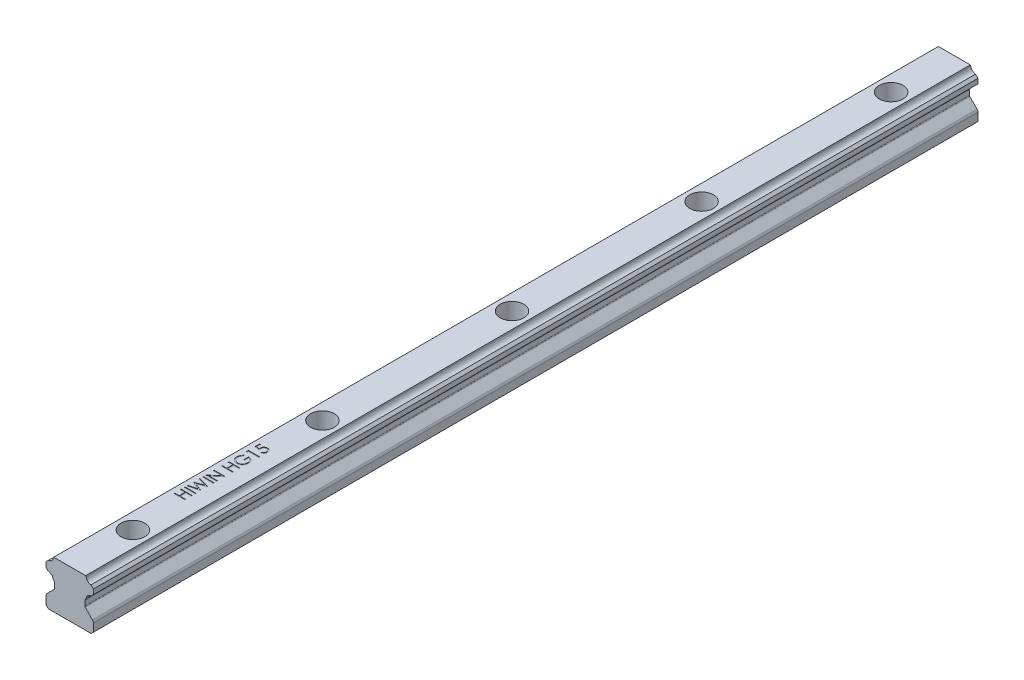
from build123d import *

# Parameters (mm, degrees)
BOSS_EXTRUDE1_DEPTH                                 = 280
CBORE_FOR_M4_HEX_SOCKET_HEAD_CAP_SCREW1_D           = 4.5
CBORE_FOR_M4_HEX_SOCKET_HEAD_CAP_SCREW1_CBORE_D     = 7.5
CBORE_FOR_M4_HEX_SOCKET_HEAD_CAP_SCREW1_CBORE_DEPTH = 5.3
LPATTERN1_COUNT                                     = 5
LPATTERN1_PITCH                                     = 60
SKETCH6_W                                           = 3.5
SKETCH6_H                                           = 0.314102564
CUT_EXTRUDE1_DEPTH                                  = 0.1


with BuildPart() as part:
    # Sketch1 → Boss-Extrude1 (new body)
    with BuildSketch(Plane.XY):
        with BuildLine():
            Line((7.5, 12.548994949), (6.730359225, 13.318635725))
            ThreePointArc((6.730359225, 13.318635725), (5.723905866, 13.746099326), (5.218323295, 14.715666114))
            ThreePointArc((5.218323295, 14.715666114), (5.180299299, 14.839173933), (5.104881891, 14.944113058))
            Line((5.104881891, 14.944113058), (5.04899495, 15))
            Line((5.04899495, 15), (-5.04899495, 15))
            Line((-5.04899495, 15), (-5.104881891, 14.944113058))
            ThreePointArc((-5.104881891, 14.944113058), (-5.180299299, 14.839173933), (-5.218323294, 14.715666114))
            ThreePointArc((-5.218323294, 14.715666114), (-5.723905866, 13.746099326), (-6.730359225, 13.318635725))
            Line((-6.730359225, 13.318635725), (-7.5, 12.548994949))
            Line((-7.5, 12.548994949), (-7.5, 11.011005051))
            Line((-7.5, 11.011005051), (-6.741857404, 10.252862454))
            ThreePointArc((-6.741857404, 10.252862454), (-5.724401564, 9.825237084), (-5.216972518, 8.845137289))
            ThreePointArc((-5.216972518, 8.845137289), (-5.179171399, 8.720266667), (-5.10319759, 8.614202641))
            Line((-5.10319759, 8.614202641), (-4.887157287, 8.398162338))
            ThreePointArc((-4.887157287, 8.398162338), (-4.800448187, 8.268392999), (-4.77, 8.115319626))
            Line((-4.77, 8.115319626), (-4.77, 6.553259018))
            ThreePointArc((-4.77, 6.553259018), (-4.800448187, 6.400185645), (-4.887157287, 6.270416306))
            Line((-4.887157287, 6.270416306), (-7.207106781, 3.950466812))
            ThreePointArc((-7.207106781, 3.950466812), (-7.423879533, 3.626043463), (-7.5, 3.243360031))
            Line((-7.5, 3.243360031), (-7.5, 0.7))
            Line((-7.5, 0.7), (-6.8, 0))
            Line((-6.8, 0), (6.8, 0))
            Line((6.8, 0), (7.5, 0.7))
            Line((7.5, 0.7), (7.5, 3.243360031))
            ThreePointArc((7.5, 3.243360031), (7.423879533, 3.626043463), (7.207106781, 3.950466812))
            Line((7.207106781, 3.950466812), (4.887157287, 6.270416306))
            ThreePointArc((4.887157287, 6.270416306), (4.800448187, 6.400185645), (4.77, 6.553259018))
            Line((4.77, 6.553259018), (4.77, 8.115319626))
            ThreePointArc((4.77, 8.115319626), (4.800448187, 8.268392999), (4.887157287, 8.398162338))
            Line((4.887157287, 8.398162338), (5.10319759, 8.614202641))
            ThreePointArc((5.10319759, 8.614202641), (5.179171399, 8.720266667), (5.216972518, 8.845137289))
            ThreePointArc((5.216972518, 8.845137289), (5.724401564, 9.825237084), (6.741857404, 10.252862454))
            Line((6.741857404, 10.252862454), (7.5, 11.011005051))
            Line((7.5, 11.011005051), (7.5, 12.548994949))
        make_face()
    extrude(amount=-BOSS_EXTRUDE1_DEPTH)

    # CBORE for M4 Hex Socket Head Cap Screw1 (through all)
    with Locations(Plane(origin=(0.291487344, 15, -3.466272926), x_dir=(-1, 0, 0), z_dir=(0, 1, 0))):
        with Locations((0.291487344, -16.533727074)):
            cbore_for_m4_hex_socket_head_cap_screw1 = CounterBoreHole(CBORE_FOR_M4_HEX_SOCKET_HEAD_CAP_SCREW1_D / 2, CBORE_FOR_M4_HEX_SOCKET_HEAD_CAP_SCREW1_CBORE_D / 2, CBORE_FOR_M4_HEX_SOCKET_HEAD_CAP_SCREW1_CBORE_DEPTH)

    # LPattern1: CBORE for M4 Hex Socket Head Cap Screw1 ×5
    with Locations(*[(0, 0, -i * LPATTERN1_PITCH) for i in range(1, LPATTERN1_COUNT)]):
        add(cbore_for_m4_hex_socket_head_cap_screw1, mode=Mode.SUBTRACT)

    # Sketch6 → Cut-Extrude1 (cut)
    with BuildSketch(Plane(origin=(0, 15, 0), x_dir=(1, 0, 0), z_dir=(0, 1, 0))):
        Polygon((-3.5, 36.403846154), (-3.5, 36.717948718), (-2.064102564, 36.717948718), (-2.064102564, 38.512820513), (-3.5, 38.512820513), (-3.5, 38.826923077), (0, 38.826923077), (0, 38.512820513), (-1.705128205, 38.512820513), (-1.705128205, 36.717948718), (0, 36.717948718), (0, 36.403846154), align=None)
        with Locations((-1.75, 39.881410256)):
            Rectangle(SKETCH6_W, SKETCH6_H)
        Polygon((-3.5, 40.576923077), (-3.5, 40.901542468), (-0.933193109, 41.586538462), (-3.5, 42.605268429), (-3.5, 42.650841346), (-0.950721154, 43.650641026), (-3.5, 44.339142628), (-3.5, 44.66025641), (0, 43.716546474), (0, 43.671674679), (-2.676883013, 42.618589744), (0, 41.552884615), (0, 41.508012821), align=None)
        with Locations((-1.75, 45.625)):
            Rectangle(SKETCH6_W, SKETCH6_H)
        Polygon((0, 46.544871795), (-3.5, 46.544871795), (-3.5, 46.610777244), (-0.745292468, 48.923076923), (-3.5, 48.923076923), (-3.5, 49.237179487), (0, 49.237179487), (0, 49.165665064), (-2.748397436, 46.858974359), (0, 46.858974359), align=None)
        Polygon((-3.5, 51.480769231), (-3.5, 51.794871795), (-2.064102564, 51.794871795), (-2.064102564, 53.58974359), (-3.5, 53.58974359), (-3.5, 53.903846154), (0, 53.903846154), (0, 53.58974359), (-1.705128205, 53.58974359), (-1.705128205, 51.794871795), (0, 51.794871795), (0, 51.480769231), align=None)
        with BuildLine():
            Line((-2.902644231, 58.076923077), (-2.647435897, 57.807692308))
            add(Edge.make_bspline(
                [(-2.647435897, 57.807692308), (-2.69328212, 57.758983227), (-2.783881335, 57.662726562), (-2.901244074, 57.50552662), (-3.002777003, 57.342170767), (-3.084772592, 57.172394867), (-3.149094254, 57.000650867), (-3.195850217, 56.829891913), (-3.225460377, 56.661223615), (-3.229016796, 56.549059313), (-3.230769231, 56.493790064)],
                knots=[0, 0, 0, 0, 1.089067066, 2.152164705, 3.18986567, 4.218445106, 5.218487318, 6.173592265, 7.100032889, 8, 8, 8, 8], degree=3))
            add(Edge.make_bspline(
                [(-3.230769231, 56.493790064), (-3.230355625, 56.459875364), (-3.229529486, 56.392133924), (-3.218985271, 56.29151198), (-3.203820407, 56.191945342), (-3.181878529, 56.093621968), (-3.15406947, 55.99635068), (-3.119284004, 55.900469793), (-3.078728771, 55.805800421), (-3.031866252, 55.713234402), (-2.980386575, 55.623493669), (-2.923337414, 55.538737672), (-2.862550889, 55.458421211), (-2.796491613, 55.384072004), (-2.725807311, 55.31519549), (-2.651770944, 55.250524789), (-2.572926872, 55.191265211), (-2.489599321, 55.138479571), (-2.403726867, 55.090811977), (-2.316037795, 55.049619777), (-2.227346143, 55.013809823), (-2.136984078, 54.986535862), (-2.045883197, 54.963434988), (-1.953566086, 54.947353752), (-1.859791669, 54.938257435), (-1.796993971, 54.936686944), (-1.765424679, 54.935897436)],
                knots=[0, 0, 0, 0, 1.028150113, 2.053633673, 3.06513288, 4.081487945, 5.106702018, 6.131327874, 7.172780699, 8.228344599, 9.276313556, 10.308389736, 11.324843658, 12.329040066, 13.321460474, 14.316307835, 15.308626991, 16.309440696, 17.305625405, 18.28535951, 19.246194545, 20.203493668, 21.145557131, 22.095268976, 23.042464743, 24, 24, 24, 24], degree=3))
            add(Edge.make_bspline(
                [(-1.765424679, 54.935897436), (-1.733154018, 54.936653631), (-1.668700816, 54.938163957), (-1.572504414, 54.947817154), (-1.477747832, 54.965772364), (-1.384282029, 54.989584114), (-1.291920993, 55.019856789), (-1.20076111, 55.057049303), (-1.110811241, 55.101355435), (-1.022964324, 55.152526704), (-0.937464192, 55.209036172), (-0.856251713, 55.271187356), (-0.780271995, 55.339084893), (-0.708415252, 55.411483836), (-0.641134974, 55.489043832), (-0.579242122, 55.572517364), (-0.521779643, 55.660735956), (-0.469378807, 55.753738745), (-0.42257144, 55.850542725), (-0.38094723, 55.949799156), (-0.346667976, 56.051827058), (-0.31872985, 56.156089724), (-0.295829559, 56.262463002), (-0.281097077, 56.371486803), (-0.270406246, 56.482359512), (-0.269624576, 56.557098144), (-0.269230769, 56.594751603)],
                knots=[0, 0, 0, 0, 0.935915162, 1.869274651, 2.799799983, 3.730201895, 4.664668062, 5.616159355, 6.583070886, 7.570012957, 8.562524459, 9.553461134, 10.53281078, 11.515274572, 12.509912756, 13.507571325, 14.526460018, 15.561318395, 16.601025881, 17.643204557, 18.680545676, 19.719612342, 20.772381578, 21.833430283, 22.908478249, 24, 24, 24, 24], degree=3))
            add(Edge.make_bspline(
                [(-0.269230769, 56.594751603), (-0.270178952, 56.640130135), (-0.272040863, 56.729238255), (-0.286546735, 56.860222075), (-0.309173205, 56.986034693), (-0.342412256, 57.106266531), (-0.384484705, 57.221353926), (-0.436513285, 57.330872414), (-0.497950569, 57.435124408), (-0.567552463, 57.533658668), (-0.645100929, 57.624132689), (-0.728035637, 57.706474768), (-0.817431068, 57.77785339), (-0.911954918, 57.840400707), (-1.012511326, 57.892097951), (-1.118540888, 57.934543829), (-1.230109213, 57.967076285), (-1.307200733, 57.980431374), (-1.346153846, 57.987179487)],
                knots=[0, 0, 0, 0, 1.130199668, 2.219330667, 3.279027493, 4.311506524, 5.322739849, 6.327972234, 7.327472899, 8.33386792, 9.329086447, 10.29244429, 11.240784345, 12.174119183, 13.111530729, 14.052100829, 15.015757696, 16, 16, 16, 16], degree=3))
            Line((-1.346153846, 57.987179487), (-1.346153846, 56.820512821))
            Line((-1.346153846, 56.820512821), (-1.705128205, 56.820512821))
            Line((-1.705128205, 56.820512821), (-1.705128205, 58.301282051))
            add(Edge.make_bspline(
                [(-1.705128205, 58.301282051), (-1.638220716, 58.299576203), (-1.507270675, 58.296237549), (-1.316300404, 58.272818634), (-1.13592871, 58.235002122), (-0.965965639, 58.18334181), (-0.806652046, 58.116466529), (-0.65782618, 58.035094001), (-0.520449499, 57.93792188), (-0.393400495, 57.828411438), (-0.280071283, 57.705511481), (-0.180465345, 57.572542861), (-0.09656273, 57.429285892), (-0.028302067, 57.275876085), (0.024971927, 57.112815651), (0.062743504, 56.939727272), (0.085373467, 56.756845671), (0.088264847, 56.631508994), (0.08974359, 56.567407853)],
                knots=[0, 0, 0, 0, 1.140356446, 2.231883559, 3.274166699, 4.278491846, 5.25512956, 6.21435461, 7.1637429, 8.11826594, 9.068280886, 10.0076534, 10.945064095, 11.891975133, 12.864533718, 13.863980011, 14.907571808, 16, 16, 16, 16], degree=3))
            add(Edge.make_bspline(
                [(0.08974359, 56.567407853), (0.089174469, 56.527897717), (0.088051978, 56.449970996), (0.080074631, 56.334880068), (0.067794054, 56.222962448), (0.049248931, 56.114234439), (0.026534277, 56.008296097), (-0.002552442, 55.905676512), (-0.036221141, 55.80598477), (-0.074516815, 55.709066784), (-0.118888472, 55.615802237), (-0.168198111, 55.52577572), (-0.222191472, 55.438489595), (-0.281802318, 55.35453843), (-0.346584778, 55.273484808), (-0.416668697, 55.195851364), (-0.491839816, 55.121203486), (-0.545218826, 55.074443023), (-0.572115385, 55.05088141)],
                knots=[0, 0, 0, 0, 1.107784379, 2.184907829, 3.233506516, 4.263428166, 5.276301166, 6.270063455, 7.25232949, 8.225834625, 9.190232166, 10.146266622, 11.1027726, 12.066435141, 13.031522626, 14.010570082, 14.99756817, 16, 16, 16, 16], degree=3))
            add(Edge.make_bspline(
                [(-0.572115385, 55.05088141), (-0.614786038, 55.016695478), (-0.699419055, 54.948891066), (-0.835018999, 54.861612909), (-0.975420859, 54.787211506), (-1.121015488, 54.726843684), (-1.271666701, 54.679705598), (-1.427181992, 54.645899345), (-1.587761622, 54.626092056), (-1.696426887, 54.623238518), (-1.751402244, 54.621794872)],
                knots=[0, 0, 0, 0, 1.023165419, 2.029347347, 3.013907458, 3.994755782, 4.975994455, 5.96558838, 6.970761222, 8, 8, 8, 8], degree=3))
            add(Edge.make_bspline(
                [(-1.751402244, 54.621794872), (-1.792568496, 54.62232711), (-1.874377804, 54.623384821), (-1.99583511, 54.636210339), (-2.115135808, 54.654611751), (-2.232182344, 54.681658827), (-2.347053012, 54.715755013), (-2.45980069, 54.758308794), (-2.570493643, 54.807852572), (-2.67836343, 54.865442289), (-2.782003044, 54.929511026), (-2.880905313, 54.999118682), (-2.973467332, 55.074802367), (-3.059903521, 55.156782462), (-3.141494975, 55.243406392), (-3.216537375, 55.336492693), (-3.286205011, 55.434631029), (-3.349159221, 55.538582169), (-3.405727075, 55.6467058), (-3.455315154, 55.758766886), (-3.496298775, 55.874724704), (-3.531072472, 55.993712261), (-3.556787635, 56.11662974), (-3.575436374, 56.242585283), (-3.588196976, 56.372235393), (-3.589223231, 56.459871423), (-3.58974359, 56.504306891)],
                knots=[0, 0, 0, 0, 1.00895651, 2.005089799, 2.991467152, 3.967318338, 4.948153826, 5.927364234, 6.919980553, 7.91976625, 8.923240147, 9.905815003, 10.88314567, 11.851989312, 12.825009789, 13.798721852, 14.781296708, 15.773896486, 16.776076962, 17.771600213, 18.775744723, 19.78957137, 20.808953803, 21.851964491, 22.910847925, 24, 24, 24, 24], degree=3))
            add(Edge.make_bspline(
                [(-3.58974359, 56.504306891), (-3.589164098, 56.540545135), (-3.588015034, 56.612401313), (-3.580050386, 56.719327046), (-3.567426505, 56.82460006), (-3.550199718, 56.92837645), (-3.526736028, 57.030302816), (-3.498657743, 57.130669522), (-3.46596592, 57.229622058), (-3.426977074, 57.326850307), (-3.382723449, 57.423008023), (-3.332910027, 57.518629864), (-3.276685022, 57.61338911), (-3.213881487, 57.707450091), (-3.145578069, 57.801405949), (-3.069821245, 57.893770591), (-2.989598489, 57.986773536), (-2.931916305, 58.04657535), (-2.902644231, 58.076923077)],
                knots=[0, 0, 0, 0, 0.985871117, 1.954866573, 2.915460327, 3.869826059, 4.81536089, 5.759505086, 6.70452669, 7.649098992, 8.607881297, 9.583363685, 10.581137262, 11.603961102, 12.659522466, 13.73993555, 14.853081303, 16, 16, 16, 16], degree=3))
        make_face()
        Polygon((-3.5, 59.449018429), (-3.5, 60.096153846), (0, 60.096153846), (0, 59.782051282), (-3.141025641, 59.782051282), (-3.141025641, 59.243589744), align=None)
        with BuildLine():
            Line((-3.5, 63.596153846), (-3.141025641, 63.596153846))
            Line((-3.141025641, 63.596153846), (-3.141025641, 62.405649038))
            Line((-3.141025641, 62.405649038), (-2.220452724, 62.217047276))
            add(Edge.make_bspline(
                [(-2.220452724, 62.217047276), (-2.230682996, 62.25410315), (-2.25050253, 62.325893046), (-2.2725083, 62.431852907), (-2.285773744, 62.53244511), (-2.287585055, 62.597720481), (-2.288461538, 62.629306891)],
                knots=[0, 0, 0, 0, 1.100273476, 2.13160584, 3.095893838, 4, 4, 4, 4], degree=3))
            add(Edge.make_bspline(
                [(-2.288461538, 62.629306891), (-2.28764354, 62.668397805), (-2.28603515, 62.745260309), (-2.269673986, 62.857544614), (-2.245976174, 62.96527195), (-2.209465207, 63.066851732), (-2.164878805, 63.163891055), (-2.108721258, 63.254723386), (-2.04315746, 63.34062356), (-1.968525078, 63.420997879), (-1.885534459, 63.493570878), (-1.795933934, 63.556634421), (-1.701678739, 63.611677196), (-1.600559725, 63.654605621), (-1.494484031, 63.689639403), (-1.382227183, 63.712740767), (-1.264785773, 63.728171477), (-1.18448027, 63.729891917), (-1.143529647, 63.730769231)],
                knots=[0, 0, 0, 0, 1.052805225, 2.070078116, 3.052532748, 4.020689046, 4.973125432, 5.925915817, 6.89216474, 7.881560752, 8.877013184, 9.857446635, 10.830895175, 11.812622661, 12.812548702, 13.836681939, 14.896847428, 16, 16, 16, 16], degree=3))
            add(Edge.make_bspline(
                [(-1.143529647, 63.730769231), (-1.115007605, 63.730103556), (-1.058348972, 63.728781204), (-0.974202158, 63.7220714), (-0.891849045, 63.709103007), (-0.811440613, 63.69190289), (-0.732901554, 63.668941583), (-0.65579213, 63.642084161), (-0.580956685, 63.608702163), (-0.508064701, 63.571694489), (-0.437950402, 63.530715464), (-0.372294905, 63.484635462), (-0.309599937, 63.436755685), (-0.251727444, 63.384438189), (-0.198452948, 63.328277796), (-0.149513072, 63.268586987), (-0.104029493, 63.205907167), (-0.063861909, 63.139251137), (-0.026898788, 63.070108867), (0.003424705, 62.997480593), (0.030535245, 62.923019908), (0.05214477, 62.845655028), (0.069077325, 62.765561217), (0.080577925, 62.682606441), (0.088954363, 62.597225771), (0.08947872, 62.539350758), (0.08974359, 62.510116186)],
                knots=[0, 0, 0, 0, 1.056393913, 2.098511576, 3.122979385, 4.141471433, 5.141222888, 6.151259816, 7.162667642, 8.172852865, 9.177685681, 10.166741883, 11.141342384, 12.097242845, 13.052202613, 14.005160326, 14.953864445, 15.917140761, 16.884916217, 17.854238259, 18.828761908, 19.81781811, 20.826036654, 21.857789401, 22.917898972, 24, 24, 24, 24], degree=3))
            add(Edge.make_bspline(
                [(0.08974359, 62.510116186), (0.089050894, 62.475242894), (0.087688097, 62.406633813), (0.073496095, 62.30610057), (0.053035464, 62.209432256), (0.022721931, 62.117043177), (-0.016971483, 62.029318648), (-0.064133263, 61.945002475), (-0.12027864, 61.865139718), (-0.184894072, 61.790276377), (-0.255892818, 61.721460371), (-0.332202561, 61.65905751), (-0.413920487, 61.604193873), (-0.500780871, 61.556670445), (-0.592629648, 61.516184815), (-0.689749822, 61.484366409), (-0.791650601, 61.45868899), (-0.861804004, 61.447825441), (-0.897435897, 61.442307692)],
                knots=[0, 0, 0, 0, 1.046872515, 2.059598001, 3.044168548, 4.012104806, 4.973680974, 5.932408326, 6.910122221, 7.900780896, 8.89867654, 9.876692837, 10.858029398, 11.85084981, 12.847361615, 13.868568023, 14.917415949, 16, 16, 16, 16], degree=3))
            Line((-0.897435897, 61.442307692), (-0.897435897, 61.756410256))
            add(Edge.make_bspline(
                [(-0.897435897, 61.756410256), (-0.86405597, 61.764133979), (-0.799897896, 61.778979402), (-0.709812799, 61.811649494), (-0.62950762, 61.851206459), (-0.558491359, 61.899340396), (-0.495464081, 61.955133792), (-0.43989307, 62.019990731), (-0.389697273, 62.092289811), (-0.347784769, 62.17267219), (-0.312479137, 62.257640252), (-0.287283878, 62.346063351), (-0.272032646, 62.436668904), (-0.270168243, 62.497671524), (-0.269230769, 62.528345353)],
                knots=[0, 0, 0, 0, 1.13623081, 2.183898708, 3.172478118, 4.09966615, 5.022692284, 5.957376522, 6.927682873, 7.937366477, 8.960015386, 9.976409503, 10.982481913, 12, 12, 12, 12], degree=3))
            add(Edge.make_bspline(
                [(-0.269230769, 62.528345353), (-0.270058415, 62.558301256), (-0.271688055, 62.617284674), (-0.284028564, 62.704132513), (-0.303533592, 62.787735767), (-0.33085902, 62.868242843), (-0.367008958, 62.945258145), (-0.411417074, 63.018672781), (-0.462975425, 63.089532607), (-0.521904738, 63.1559727), (-0.586881759, 63.216808942), (-0.656357238, 63.270565902), (-0.730474586, 63.315342595), (-0.807947606, 63.353076763), (-0.889626199, 63.381730046), (-0.975127364, 63.402171031), (-1.064662347, 63.414174089), (-1.125731657, 63.415825269), (-1.156850962, 63.416666667)],
                knots=[0, 0, 0, 0, 1.027268864, 2.022700798, 3.002744649, 3.968653148, 4.933396556, 5.915045722, 6.907600446, 7.935526002, 8.956456544, 9.95700807, 10.942805781, 11.92166854, 12.907987664, 13.905483474, 14.932689774, 16, 16, 16, 16], degree=3))
            add(Edge.make_bspline(
                [(-1.156850962, 63.416666667), (-1.184930032, 63.416028195), (-1.239659043, 63.414783746), (-1.320009695, 63.404010642), (-1.396158478, 63.386014341), (-1.468436727, 63.360391264), (-1.536613353, 63.328412845), (-1.600538112, 63.288262971), (-1.660812066, 63.241651258), (-1.715884112, 63.187233139), (-1.766793088, 63.12803749), (-1.810034281, 63.062543866), (-1.846807397, 62.992500701), (-1.876936465, 62.917778197), (-1.900936575, 62.838284311), (-1.917523378, 62.753976228), (-1.92744867, 62.664834733), (-1.928795087, 62.603859089), (-1.929487179, 62.572516026)],
                knots=[0, 0, 0, 0, 1.045723156, 2.038222538, 3.013889863, 3.95567481, 4.890389958, 5.81331128, 6.76251276, 7.723027653, 8.692928204, 9.666105983, 10.639751036, 11.635719707, 12.66315958, 13.728667616, 14.832476222, 16, 16, 16, 16], degree=3))
            add(Edge.make_bspline(
                [(-1.929487179, 62.572516026), (-1.928906588, 62.545387097), (-1.927707815, 62.489372742), (-1.918881318, 62.403449915), (-1.904642024, 62.313158192), (-1.885055776, 62.218843696), (-1.859424699, 62.120223188), (-1.828710199, 62.017504787), (-1.7919882, 61.910472521), (-1.764255986, 61.838354796), (-1.75, 61.801282051)],
                knots=[0, 0, 0, 0, 0.817624296, 1.688186739, 2.600797293, 3.572016777, 4.590301741, 5.671205678, 6.80286297, 8, 8, 8, 8], degree=3))
            Line((-1.75, 61.801282051), (-3.5, 62.16025641))
            Line((-3.5, 62.16025641), (-3.5, 63.596153846))
        make_face()
    extrude(amount=-CUT_EXTRUDE1_DEPTH, mode=Mode.SUBTRACT)


solid = part.part
